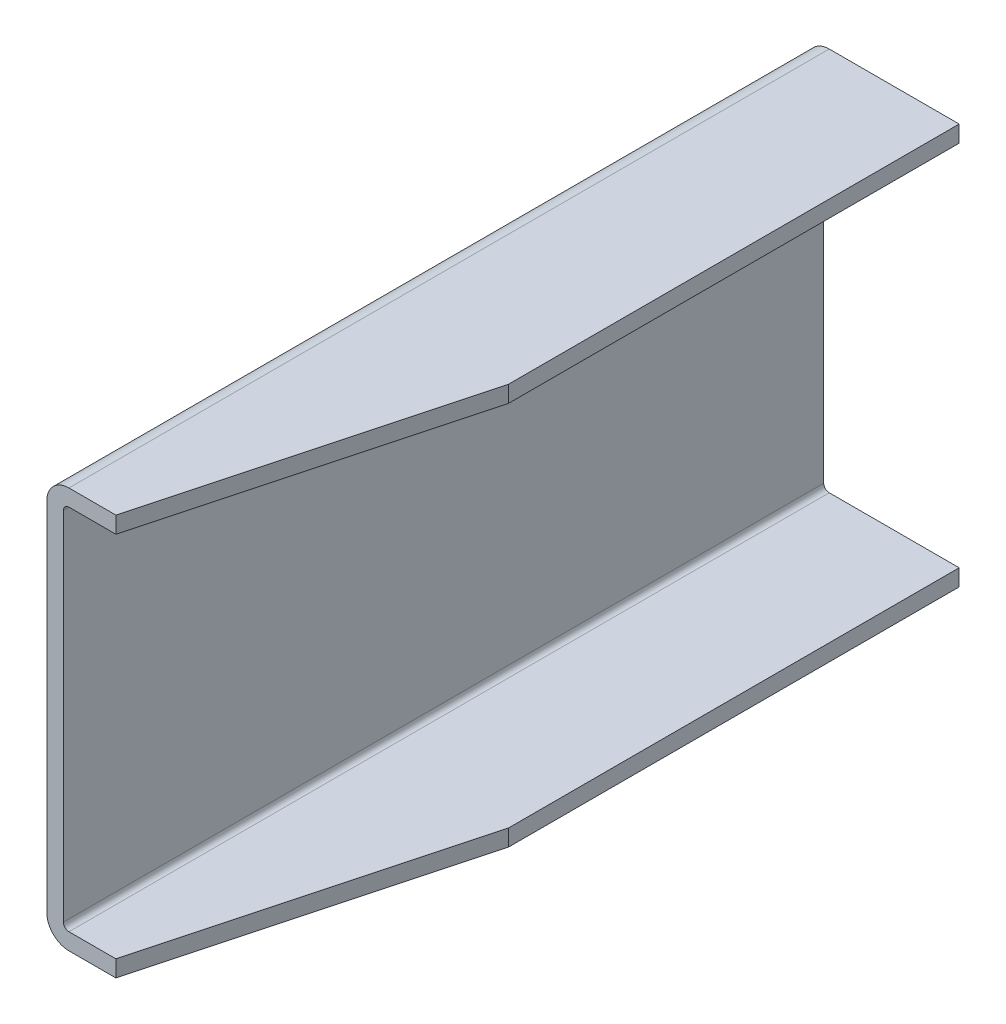
SolidWorks part; units mm, degrees
material "1023 碳钢板 (SS)"
ref_plane "前视基准面" through (0, 0, 0) normal (0, 0, 1) x (1, 0, 0)
ref_plane "上视基准面" through (0, 0, 0) normal (0, 1, 0) x (1, 0, 0)
ref_plane "右视基准面" through (0, 0, 0) normal (1, 0, 0) x (0, 0, -1)
sketch "草图1" plane through (0, 0, 0) normal (0, 0, 1) x (1, 0, 0)
  line L0 (0, 0) -> (-47, 0)
  line L1 (-55, -8) -> (-55, -137)
  line L2 (-47, -145) -> (0, -145)
  line L3 (0, -6) -> (-47, -6)
  line L4 (-49, -8) -> (-49, -137)
  line L5 (-47, -139) -> (0, -139)
  line L6 (0, 0) -> (0, -6)
  line L7 (0, -139) -> (0, -145)
  arc A0 (-55, -137) -> (-47, -145) centre (-47, -137) ccw
  arc A1 (-47, 0) -> (-55, -8) centre (-47, -8) ccw
  arc A2 (-47, -6) -> (-49, -8) centre (-47, -8) ccw
  arc A3 (-49, -137) -> (-47, -139) centre (-47, -137) ccw
  point P7 (-55, -145)
  point P10 (-55, 0)
  dimension "D3" = 8
  dimension "D1" = 55
  dimension "D2" = 145
  dimension "D4" = 6
extrude "凸台-拉伸1" add sketch "草图1" along normal blind 275
sketch "草图2" plane through (0, 0, 0) normal (0, 1, 0) x (1, 0, 0)
  line L0 (0, -163) -> (-30, -275)
  line L1 (0, -275) -> (0, 0) construction
  line L2 (0, -275) -> (-47, -275) construction
  line L3 (-30, -275) -> (0, -275)
  line L4 (0, -275) -> (0, -163)
  dimension "D1" = 112
  dimension "D2" = 30
extrude "切除-拉伸1" cut sketch "草图2" against normal blind 275
